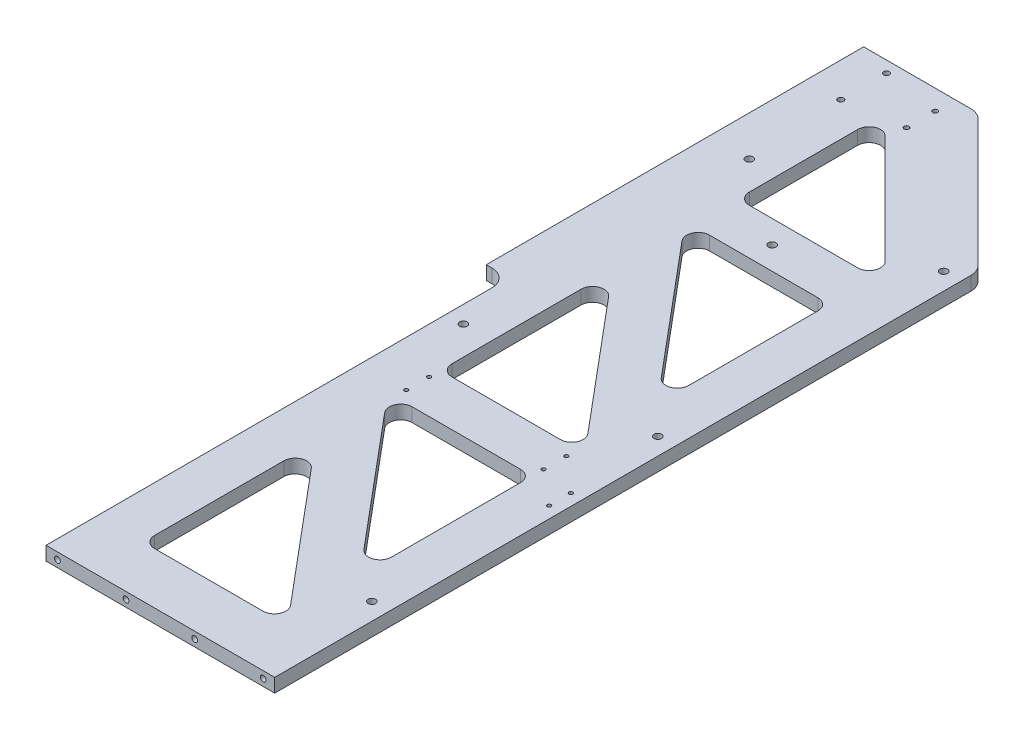
SolidWorks part; units mm, degrees
material "A6061"
ref_plane "前基準面" through (0, 0, 0) normal (0, 0, 1) x (1, 0, 0)
ref_plane "上基準面" through (0, 0, 0) normal (0, 1, 0) x (1, 0, 0)
ref_plane "右基準面" through (0, 0, 0) normal (1, 0, 0) x (0, 0, -1)
sketch "草图1" plane through (0, 0, 0) normal (0, 1, 0) x (1, 0, 0)
  line L1 (-110, -165) -> (110, -165)
  line L2 (-110, -165) -> (-110, 165)
  line L3 (-110, 165) -> (110, 165)
  line L4 (110, -165) -> (110, 165)
  line L5 (-110, -165) -> (110, 165) construction
  line L6 (-110, 165) -> (110, -165) construction
  point P0 (0, 0)
  dimension "D1" = 220
  dimension "D2" = 330
extrude "凸台-拉伸1" add sketch "草图1" along normal mid plane 12
sketch "草图2" plane through (0, 6, 0) normal (0, 1, 0) x (1, 0, 0)
  line L0 (110, 165) -> (-110, 165) construction
  line L1 (110, -165) -> (-90, -165)
  line L2 (110, -165) -> (110, -570)
  line L3 (110, -570) -> (-90, -570)
  line L4 (-90, -165) -> (-90, -570)
  dimension "D1" = 200
  dimension "D2" = 735
extrude "凸台-拉伸2" add sketch "草图2" against normal up to surface (12 mm away) up to face at (0, -6, 0)
chamfer "倒角1" distance 120 angle 45 1 edges at (110, 0, -165)
fillet "圆角2" radius 15 3 edges at (-10, 0, -165) (110, 0, -45)
sketch "草图7" plane through (0, 6, 0) normal (0, 1, 0) x (1, 0, 0)
  line L0 (-34.7477, -45) -> (60, -45)
  line L1 (70, -55) -> (70, -167.916)
  line L2 (52.3396, -174.3438) -> (-42.4082, -61.4279)
  line L3 (-32.3396, -135.6562) -> (62.4082, -248.5721)
  line L4 (54.7477, -265) -> (-40, -265)
  line L5 (105.6066, 49.3934) -> (-5.6066, 160.6066) construction
  line L6 (-50, -255) -> (-50, -142.084)
  line L7 (-16.2132, 165) -> (-110, 165) construction
  line L9 (110, -570) -> (110, 38.7868) construction
  line L10 (-90, -180) -> (-90, -570) construction
  line L13 (-34.7477, -305) -> (60, -305)
  line L14 (70, -315) -> (70, -427.916)
  line L15 (52.3396, -434.3438) -> (-42.4082, -321.4279)
  line L16 (-32.3396, -395.6562) -> (62.4082, -508.5721)
  line L17 (54.7477, -525) -> (-40, -525)
  line L18 (-50, -515) -> (-50, -402.084)
  line L20 (-50, 99.7477) -> (-50, 5)
  line L21 (-40, -5) -> (54.7477, -5)
  line L22 (61.8188, 12.0711) -> (-32.9289, 106.8188)
  arc A0 (62.4082, -248.5721) -> (54.7477, -265) centre (54.7477, -255) cw
  arc A1 (-32.3396, -135.6562) -> (-50, -142.084) centre (-40, -142.084) ccw
  arc A2 (-40, -265) -> (-50, -255) centre (-40, -255) cw
  arc A3 (60, -45) -> (70, -55) centre (60, -55) cw
  arc A4 (70, -167.916) -> (52.3396, -174.3438) centre (60, -167.916) cw
  arc A5 (-34.7477, -45) -> (-42.4082, -61.4279) centre (-34.7477, -55) ccw
  arc A6 (62.4082, -508.5721) -> (54.7477, -525) centre (54.7477, -515) cw
  arc A7 (-32.3396, -395.6562) -> (-50, -402.084) centre (-40, -402.084) ccw
  arc A8 (-40, -525) -> (-50, -515) centre (-40, -515) cw
  arc A9 (60, -305) -> (70, -315) centre (60, -315) cw
  arc A10 (70, -427.916) -> (52.3396, -434.3438) centre (60, -427.916) cw
  arc A11 (-34.7477, -305) -> (-42.4082, -321.4279) centre (-34.7477, -315) ccw
  arc A12 (-50, 99.7477) -> (-32.9289, 106.8188) centre (-40, 99.7477) cw
  arc A13 (54.7477, -5) -> (61.8188, 12.0711) centre (54.7477, 5) ccw
  arc A14 (-50, 5) -> (-40, -5) centre (-40, 5) ccw
extrude "切除-拉伸3" cut sketch "草图7" against normal up to surface (12 mm away)
hole_wizard "M6 螺纹孔1" positions "草图11" profile "草图10" tap size "M6" standard "GB"
sketch "草图11" plane through (0, 0, 570) normal (0, 0, 1) x (1, 0, 0)
  line L0 (10, 6) -> (10, -6) construction
  line L1 (-90, 6) -> (110, 6) construction
  line L2 (-90, -6) -> (110, -6) construction
  line L4 (-90, 0) -> (-80, 0) construction
  line L5 (-90, -6) -> (-90, 6) construction
  point P0 (-80, 0)
  point P2 (-20, 0)
  point P13 (40, 0)
  point P14 (100, 0)
  dimension "D1" = 60
  dimension "D2" = 60
sketch "草图10" plane through (-80, 0, 570) normal (1, 0, 0) x (0, -1, 0)
  line L0 (0, 0) -> (0, 18.5022)
  line L1 (0, 18.5022) -> (2.5, 17)
  line L2 (2.5, 17) -> (2.5, 0)
  line L5 (2.5, 0) -> (0, 0)
  line L10 (0, 18.5022) -> (-2.5, 17) construction
  line L11 (0, -6.35) -> (0, 107.95) construction
  dimension "螺纹孔钻头直径" = 5
  dimension "螺纹孔钻头深度" = 17
  dimension "导头角度" = 118
cosmetic thread "孔螺蚊线9" parameters "D1"=12, "D2"=6
cosmetic thread "孔螺蚊线10" parameters "D1"=12, "D2"=6
cosmetic thread "孔螺蚊线11" parameters "D1"=12, "D2"=6
cosmetic thread "孔螺蚊线12" parameters "D1"=12, "D2"=6
hole_wizard "M6 螺纹孔2" positions "草图13" profile "草图12" tap size "M6" standard "GB"
sketch "草图13" plane through (-110, 0, 0) normal (-1, 0, 0) x (0, 0, 1)
  line L0 (0, 6) -> (0, -6) construction
  line L1 (-165, 6) -> (165, 6) construction
  line L2 (-165, -6) -> (165, -6) construction
  point P0 (-150, 0)
  point P20 (-90, 0)
  point P21 (-30, 0)
  point P22 (30, 0)
  point P23 (90, 0)
  point P24 (150, 0)
  dimension "D1" = 6
  dimension "D2" = 60
sketch "草图12" plane through (-110, 0, -150) normal (0, 1, 0) x (0, 0, 1)
  line L0 (0, 0) -> (0, 18.5022)
  line L1 (0, 18.5022) -> (2.5, 17)
  line L2 (2.5, 17) -> (2.5, 0)
  line L5 (2.5, 0) -> (0, 0)
  line L10 (0, 18.5022) -> (-2.5, 17) construction
  line L11 (0, -6.35) -> (0, 107.95) construction
  dimension "螺纹孔钻头直径" = 5
  dimension "螺纹孔钻头深度" = 17
  dimension "导头角度" = 118
cosmetic thread "孔螺蚊线5" parameters "D1"=12, "D2"=6
cosmetic thread "孔螺蚊线6" parameters "D1"=12, "D2"=6
cosmetic thread "孔螺蚊线7" parameters "D1"=12, "D2"=6
cosmetic thread "孔螺蚊线8" parameters "D1"=12, "D2"=6
cosmetic thread "孔螺蚊线17" parameters "D1"=12, "D2"=6
cosmetic thread "孔螺蚊线18" parameters "D1"=12, "D2"=6
hole_wizard "M6 间隙孔1" positions "草图14" profile "草图15" hole size "M6" standard "GB"
sketch "草图14" plane through (0, 6, 0) normal (0, 1, 0) x (1, 0, 0)
  line L0 (10, -570) -> (10, -112.3238) construction
  line L1 (-90, -570) -> (110, -570) construction
  line L3 (110, -570) -> (110, 38.7868) construction
  point P0 (95, 30)
  point P7 (-75, 30)
  point P8 (-75, -220)
  point P10 (95, -220)
  point P11 (95, -470)
  point P22 (-75, -470) [skipped]
  dimension "D3" = 15
  dimension "D4" = 250
  dimension "D5" = 100
  dimension "D1" = 2
  dimension "D2" = 3
sketch "草图15" plane through (95, 6, -30) normal (1, 0, 0) x (0, 0, 1)
  line L0 (0, 0) -> (0, 12)
  line L1 (0, 12) -> (3.3, 12)
  line L2 (3.3, 12) -> (3.3, 0)
  line L5 (3.3, 0) -> (0, 0)
  line L11 (0, -6.35) -> (0, 107.95) construction
  dimension "通孔孔直径" = 6.6
  dimension "通孔孔深度" = 12
hole_wizard "M6 间隙孔2" positions "草图16" profile "草图17" hole size "M6" standard "GB" end condition through all
sketch "草图16" plane through (0, 6, 0) normal (0, 1, 0) x (1, 0, 0)
  line L0 (0, -5) -> (0, -45) construction
  line L1 (-40, -5) -> (54.7477, -5) construction
  line L2 (60, -45) -> (-34.7477, -45) construction
  point P0 (0, -25)
sketch "草图17" plane through (0, 6, 25) normal (1, 0, 0) x (0, 0, 1)
  line L0 (0, 0) -> (0, 12)
  line L1 (0, 12) -> (3.3, 12)
  line L2 (3.3, 12) -> (3.3, 0)
  line L5 (3.3, 0) -> (0, 0)
  line L11 (0, -6.35) -> (0, 107.95) construction
  dimension "通孔孔直径" = 6.6
  dimension "通孔孔深度" = 12
hole_wizard "M6 螺纹孔3" positions "草图18" profile "草图19" tap size "M6" standard "GB" end condition through all
sketch "草图18" plane through (0, 6, 0) normal (0, 1, 0) x (1, 0, 0)
  line L0 (-16.2132, 165) -> (-110, 165) construction
  line L1 (-110, 165) -> (-110, -165) construction
  point P0 (-80, 155)
  point P2 (-80, 115)
  dimension "D1" = 10
  dimension "D2" = 40
  dimension "D3" = 30
sketch "草图19" plane through (-80, 6, -155) normal (1, 0, 0) x (0, 0, 1)
  line L0 (0, 0) -> (0, 12)
  line L1 (0, 12) -> (2.5, 12)
  line L2 (2.5, 12) -> (2.5, 0)
  line L5 (2.5, 0) -> (0, 0)
  line L11 (0, -6.35) -> (0, 107.95) construction
  dimension "通孔螺纹孔钻头直径" = 5
  dimension "通孔螺纹孔钻头深度" = 12
cosmetic thread "孔螺蚊线13" parameters "D2"=6
cosmetic thread "孔螺蚊线14" parameters "D2"=6
hole_wizard "M5 螺纹孔1" positions "草图20" profile "草图21" tap size "M5" standard "GB" end condition through all
sketch "草图20" plane through (0, 6, 0) normal (0, 1, 0) x (1, 0, 0)
  line L0 (-16.2132, 165) -> (-110, 165) construction
  line L1 (-110, 165) -> (-110, -165) construction
  point P0 (-30, 147.5)
  point P2 (-30, 122.5)
  dimension "D1" = 25
  dimension "D2" = 17.5
  dimension "D3" = 80
sketch "草图21" plane through (-30, 6, -147.5) normal (1, 0, 0) x (0, 0, 1)
  line L0 (0, 0) -> (0, 12)
  line L1 (0, 12) -> (2.1, 12)
  line L2 (2.1, 12) -> (2.1, 0)
  line L5 (2.1, 0) -> (0, 0)
  line L11 (0, -6.35) -> (0, 107.95) construction
  dimension "通孔螺纹孔钻头直径" = 4.2
  dimension "通孔螺纹孔钻头深度" = 12
cosmetic thread "孔螺蚊线15" parameters "D2"=5
cosmetic thread "孔螺蚊线16" parameters "D2"=5
hole_wizard "M4 螺纹孔1" positions "草图22" profile "草图23" tap size "M4" standard "GB" end condition through all
sketch "草图22" plane through (0, 6, 0) normal (0, 1, 0) x (1, 0, 0)
  line L0 (-90, -570) -> (110, -570) construction
  line L1 (110, -570) -> (110, 38.7868) construction
  point P0 (100, -320)
  point P2 (100, -301)
  dimension "D1" = 19
  dimension "D2" = 250
  dimension "D3" = 10
sketch "草图23" plane through (100, 6, 320) normal (1, 0, 0) x (0, 0, 1)
  line L0 (0, 0) -> (0, 12)
  line L1 (0, 12) -> (1.65, 12)
  line L2 (1.65, 12) -> (1.65, 0)
  line L5 (1.65, 0) -> (0, 0)
  line L11 (0, -6.35) -> (0, 107.95) construction
  dimension "通孔螺纹孔钻头直径" = 3.3
  dimension "通孔螺纹孔钻头深度" = 12
cosmetic thread "孔螺蚊线19" parameters "D2"=4
cosmetic thread "孔螺蚊线20" parameters "D2"=4
hole_wizard "M4 螺纹孔2" positions "草图24" profile "草图25" tap size "M4" standard "GB" end condition through all
sketch "草图24" plane through (0, 6, 0) normal (0, 1, 0) x (1, 0, 0)
  line L0 (10, -570) -> (10, -45) construction
  line L1 (-90, -570) -> (110, -570) construction
  line L3 (10, -45) -> (10, -525) construction
  line L6 (-40, -525) -> (54.7477, -525) construction
  line L7 (10, -285) -> (-58.57, -285) construction
  line L8 (-40, -265) -> (54.7477, -265) construction
  point P0 (-50, -275)
  point P18 (70, -275)
  point P23 (70, -295)
  point P24 (-50, -295)
  dimension "D1" = 120
  dimension "D2" = 20
  dimension "D3" = 10
sketch "草图25" plane through (-50, 6, 275) normal (1, 0, 0) x (0, 0, 1)
  line L0 (0, 0) -> (0, 12)
  line L1 (0, 12) -> (1.65, 12)
  line L2 (1.65, 12) -> (1.65, 0)
  line L5 (1.65, 0) -> (0, 0)
  line L11 (0, -6.35) -> (0, 107.95) construction
  dimension "通孔螺纹孔钻头直径" = 3.3
  dimension "通孔螺纹孔钻头深度" = 12
cosmetic thread "孔螺蚊线21" parameters "D2"=4
cosmetic thread "孔螺蚊线22" parameters "D2"=4
cosmetic thread "孔螺蚊线23" parameters "D2"=4
cosmetic thread "孔螺蚊线24" parameters "D2"=4
equation "\"D3@草图7\"=\"D2@草图7\""
